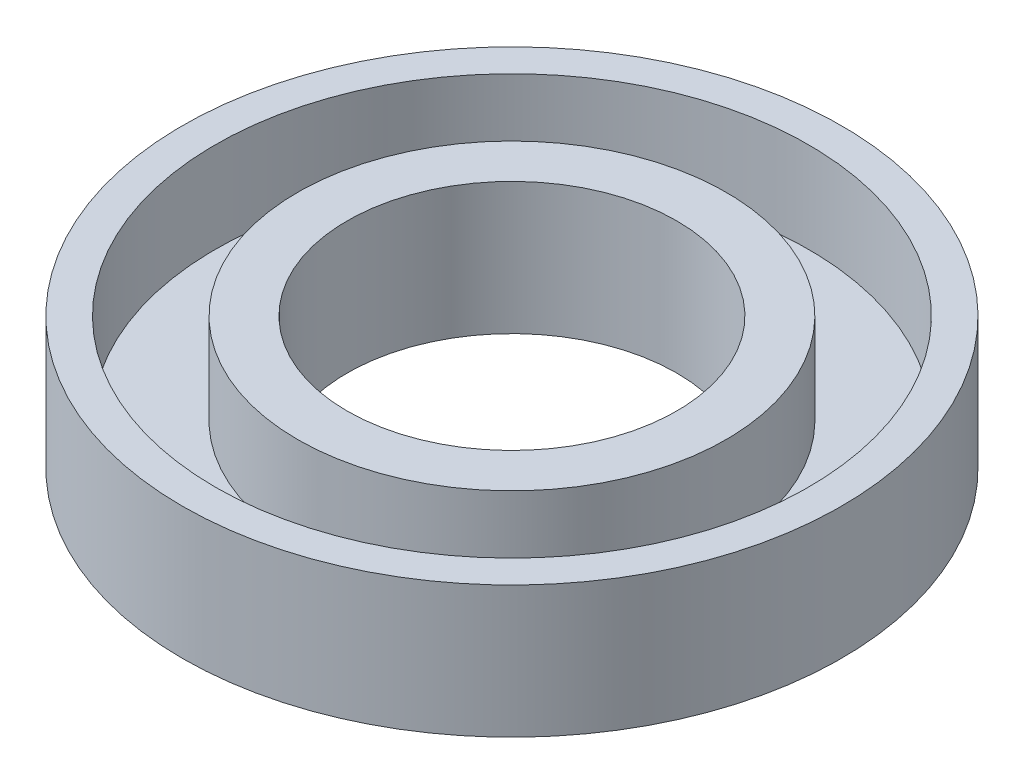
from build123d import *

# Parameters (mm, degrees)
SKETCH1_R           = 20
SKETCH1_R_2         = 10
BOSS_EXTRUDE1_DEPTH = 8
SKETCH2_R           = 18
SKETCH2_R_2         = 13
CUT_EXTRUDE1_DEPTH  = 5.5


with BuildPart() as part:
    # Sketch1 → Boss-Extrude1 (new body)
    with BuildSketch(Plane(origin=(0, 0, 0), x_dir=(1, 0, 0), z_dir=(0, 1, 0))):
        with Locations(Location((0, 0, 0), (0, 0, 270))):
            Circle(SKETCH1_R)
        with Locations(Location((0, 0, 0), (0, 0, 270))):
            Circle(SKETCH1_R_2, mode=Mode.SUBTRACT)
    extrude(amount=BOSS_EXTRUDE1_DEPTH)

    # Sketch2 → Cut-Extrude1 (cut)
    with BuildSketch(Plane(origin=(0, 8, 0), x_dir=(1, 0, 0), z_dir=(0, 1, 0))):
        with Locations(Location((0, 0, 0), (0, 0, 270))):
            Circle(SKETCH2_R)
        with Locations(Location((0, 0, 0), (0, 0, 270))):
            Circle(SKETCH2_R_2, mode=Mode.SUBTRACT)
    extrude(amount=-CUT_EXTRUDE1_DEPTH, mode=Mode.SUBTRACT)


solid = part.part
